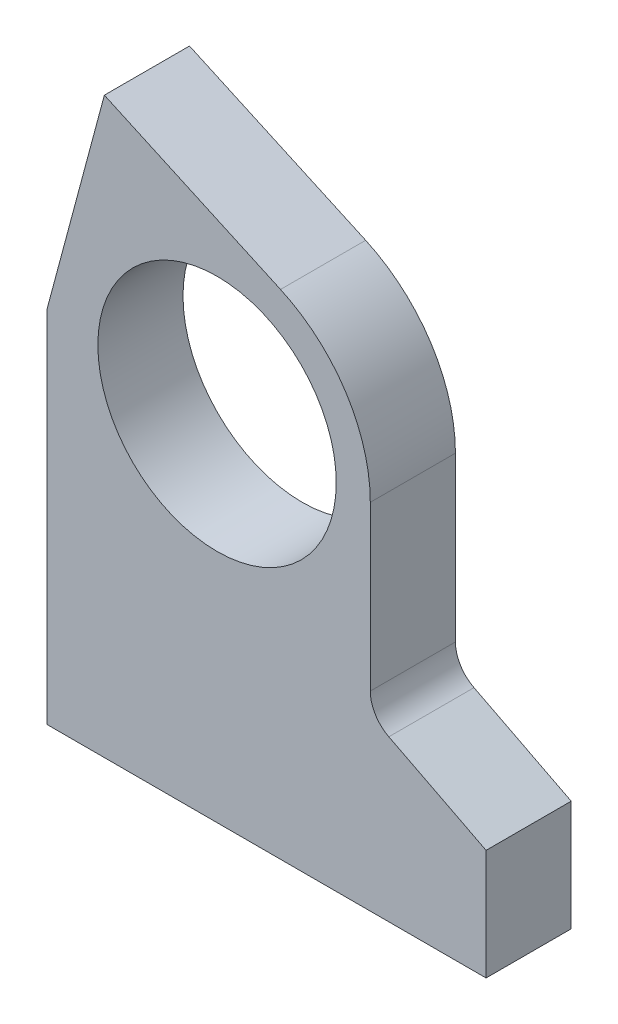
SolidWorks part; units mm, degrees
material "普通碳钢"
ref_plane "前视" through (0, 0, 0) normal (0, 0, 1) x (1, 0, 0)
ref_plane "上视" through (0, 0, 0) normal (0, 1, 0) x (1, 0, 0)
ref_plane "右视" through (0, 0, 0) normal (1, 0, 0) x (0, 0, -1)
sketch "草图1" plane through (0, 0, 0) normal (0, 0, 1) x (1, 0, 0)
  line L0 (-248.6675, 0) -> (296.7129, 0) construction
  line L1 (0, 203.5438) -> (0, -193.8048) construction
  line L2 (129, 0) -> (129, 10)
  line L3 (129, 10) -> (100.4482, 24.596)
  line L4 (95, 81.5) -> (95, 33.5)
  line L6 (16.9076, 146) -> (0, 82.9)
  line L7 (0, -22.47) -> (0, 82.9)
  line L8 (16.9076, 146) -> (68.6391, 122.4583)
  line L9 (129, 0) -> (129, -22.47)
  line L10 (129, -22.47) -> (0, -22.47)
  circle A0 centre (50, 81.5) radius 35
  arc A1 (95, 81.5) -> (68.6391, 122.4583) centre (50, 81.5) ccw
  arc A2 (95, 33.5) -> (100.4482, 24.596) centre (105, 33.5) ccw
  dimension "D1" = 70
  dimension "D2" = 90
  dimension "D6" = 20
  dimension "D3" = 50
  dimension "D4" = 81.5
  dimension "D5" = 10
  dimension "D7" = 48
  dimension "D13" = 22.47
extrude "凸台-拉伸1" add sketch "草图1" along normal blind 25
